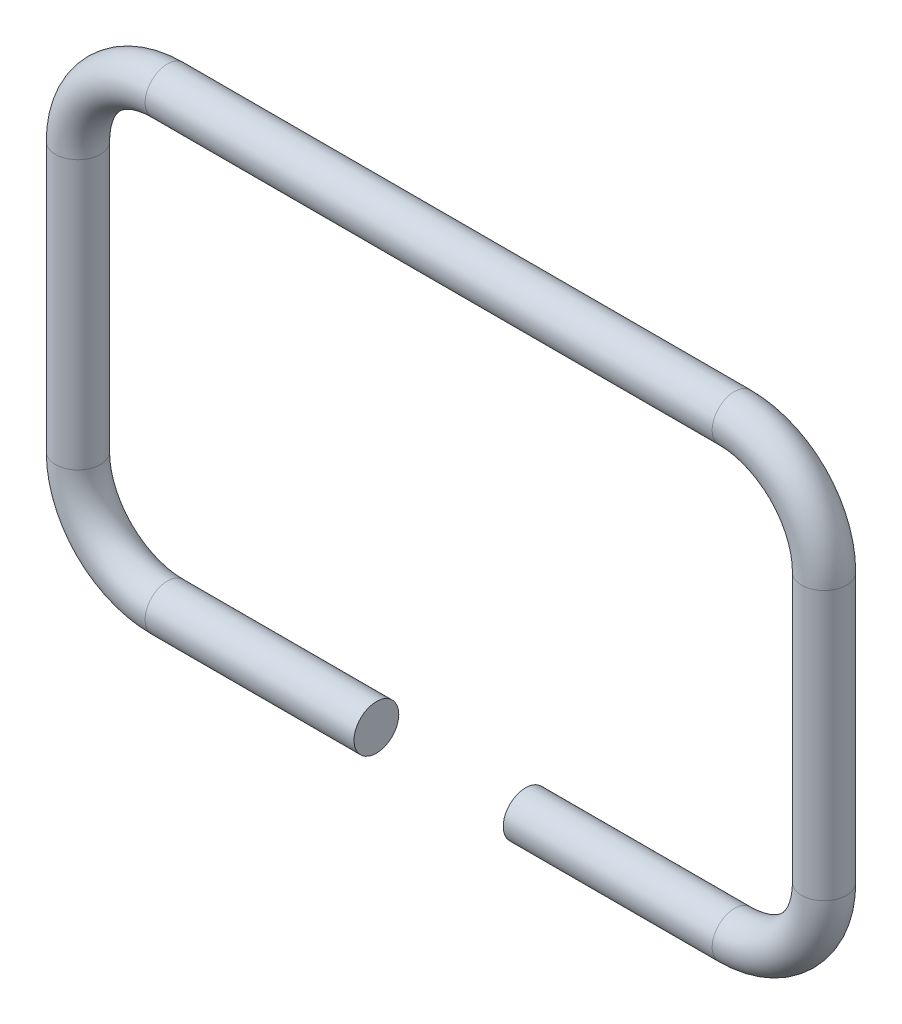
from build123d import *

# Parameters (mm, degrees)
SKETCH2_R = 7.5


with BuildPart() as part:
    # Sweep1: sweep along a path in Sketch1
    with BuildLine(Plane.XY) as sweep1_path:
        Line((0, 0), (70, 0))
        ThreePointArc((70, 0), (91.213203436, 8.786796564), (100, 30))
        Line((100, 30), (100, 120))
        ThreePointArc((100, 120), (91.213203436, 141.213203436), (70, 150))
        Line((70, 150), (-120, 150))
        ThreePointArc((-120, 150), (-141.213203436, 141.213203436), (-150, 120))
        Line((-150, 120), (-150, 30))
        ThreePointArc((-150, 30), (-141.213203436, 8.786796564), (-120, 0))
        Line((-120, 0), (-50, 0))
    # Sketch2 → Sweep1 (sweep)
    with BuildSketch(Plane(origin=(0, 0, 0), x_dir=(0, 0, -1), z_dir=(1, 0, 0))):
        Circle(SKETCH2_R)
    sweep(path=sweep1_path.line)


solid = part.part
